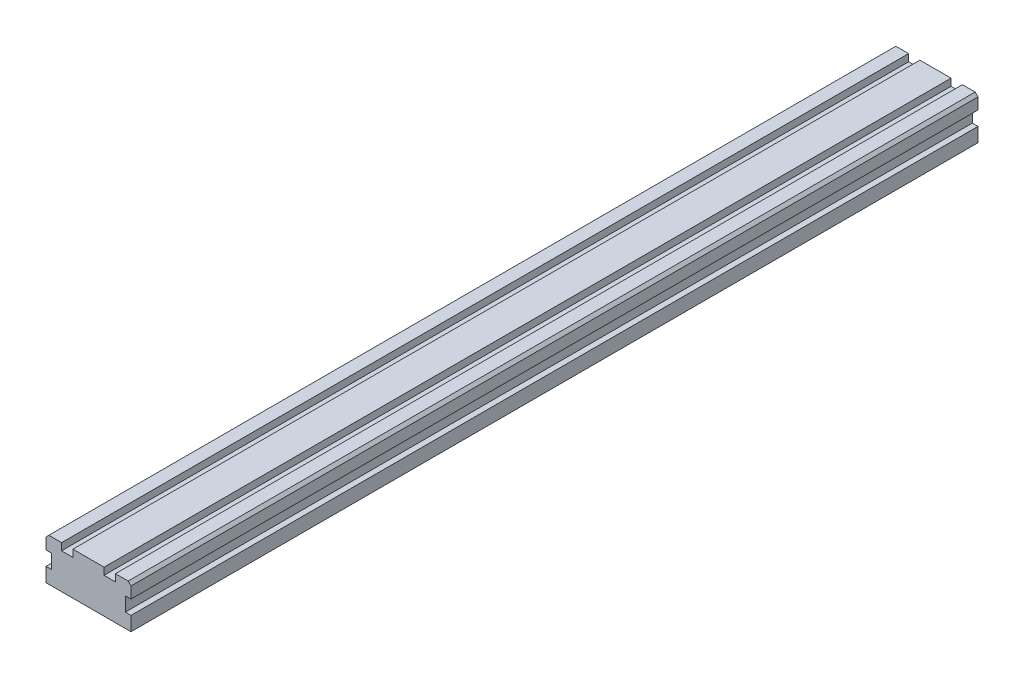
from build123d import *

# Parameters (mm, degrees)
SKETCH1_W           = 60
SKETCH1_H           = 30
BOSS_EXTRUDE1_DEPTH = 299
SKETCH2_W           = 8
SKETCH2_H           = 10
CUT_EXTRUDE1_DEPTH  = 646
CHAMFER1_SIZE       = 2


with BuildPart() as part:
    # Sketch1 → Boss-Extrude1 (new, symmetric)
    with BuildSketch(Plane.XY):
        with Locations((720, 45)):
            Rectangle(SKETCH1_W, SKETCH1_H)
    extrude(amount=BOSS_EXTRUDE1_DEPTH, both=True)

    # Sketch2 → Cut-Extrude1 (cut)
    with BuildSketch(Plane(origin=(0, 0, -299), x_dir=(-1, 0, 0), z_dir=(0, 0, -1))):
        with Locations((-735, 60)):
            Rectangle(SKETCH2_W, SKETCH2_H)
        with Locations((-750, 45)):
            Rectangle(SKETCH2_W, SKETCH2_H)
        with Locations((-690, 45)):
            Rectangle(SKETCH2_W, SKETCH2_H)
        with Locations((-705, 60)):
            Rectangle(SKETCH2_W, SKETCH2_H)
    extrude(amount=-CUT_EXTRUDE1_DEPTH, mode=Mode.SUBTRACT)

    # Chamfer1
    chamfer1_edges = [part.edges().sort_by_distance(p)[0] for p in [
        (690, 60, 0),
        (750, 60, 0),
    ]]
    chamfer(chamfer1_edges, length=CHAMFER1_SIZE)


solid = part.part
